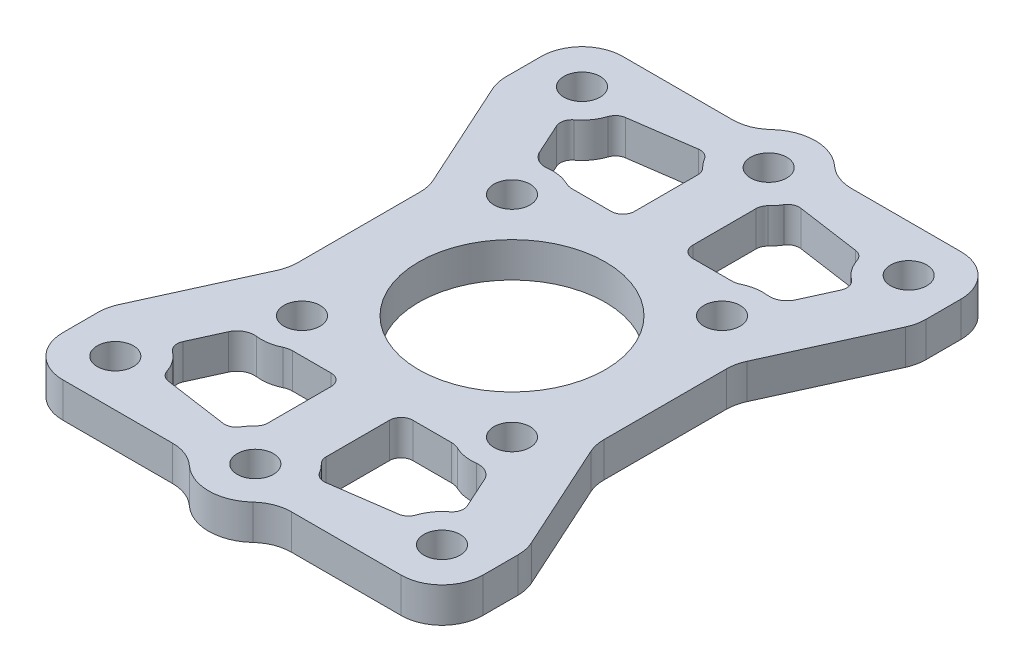
SolidWorks part; units mm, degrees
material "Thornel Mat VMA"
ref_plane "前视基准面" through (0, 0, 0) normal (0, 0, 1) x (1, 0, 0)
ref_plane "上视基准面" through (0, 0, 0) normal (0, 1, 0) x (1, 0, 0)
ref_plane "右视基准面" through (0, 0, 0) normal (1, 0, 0) x (0, 0, -1)
other "Configuration Table"
sketch "草图3" plane through (0, 0, 0) normal (0, 1, 0) x (1, 0, 0)
  line L0 (10, -34.1992) -> (10, 52.6309) construction
  line L1 (0, 0) -> (31.1432, 0) construction
  line L6 (-14, 20) -> (14, 20) construction
  line L7 (-14, 20) -> (-14, -20) construction
  line L8 (-14, -20) -> (14, -20) construction
  line L9 (14, 20) -> (14, -20) construction
  line L10 (-14, 20) -> (14, -20) construction
  line L11 (-14, -20) -> (14, 20) construction
  line L12 (-18, -24) -> (18, -24)
  line L13 (-18, -24) -> (-18, 24)
  line L14 (-18, 24) -> (18, 24)
  line L15 (18, -24) -> (18, 24)
  line L16 (-18, -24) -> (18, 24) construction
  line L17 (-18, 24) -> (18, -24) construction
  line L18 (6, 62.0596) -> (6, -48.8242) construction
  line L19 (0, 0) -> (0, -41.7674) construction
  line L21 (-9, 9) -> (9, 9) construction
  line L22 (-9, 9) -> (-9, -9) construction
  line L23 (-9, -9) -> (9, -9) construction
  line L24 (9, 9) -> (9, -9) construction
  line L25 (-9, 9) -> (9, -9) construction
  line L26 (-9, -9) -> (9, 9) construction
  circle A7 centre (14, 20) radius 1.55
  circle A8 centre (-14, 20) radius 1.55
  circle A9 centre (-14, -20) radius 1.55
  circle A10 centre (14, -20) radius 1.55
  circle A15 centre (0, 22) radius 1.55
  circle A17 centre (0, 22) radius 4
  circle A19 centre (0, -22) radius 1.55
  circle A20 centre (0, -22) radius 4
  circle A30 centre (9, 9) radius 1.55
  circle A31 centre (-9, 9) radius 1.55
  circle A32 centre (-9, -9) radius 1.55
  circle A33 centre (9, -9) radius 1.55
  circle A34 centre (0, 0) radius 8
  point P14 (0, 0)
  point P42 (0, 0)
  dimension "D2" = 6
  dimension "D4" = 16
  dimension "D9" = 3.1
  dimension "D12" = 4
  dimension "D13" = 8
  dimension "D14" = 2
  dimension "D3" = 18
  dimension "D6" = 10
  dimension "D7" = 4
  dimension "D8" = 40
  dimension "D10" = 28
  dimension "D11" = 4
extrude "凸台-拉伸1" add sketch "草图3" along normal blind 3
sketch "草图4" plane through (0, 3, 0) normal (0, 1, 0) x (1, 0, 0)
  line L17 (-14, 20) -> (0, 22) construction
  line L32 (0, 22) -> (14, 20) construction
  line L33 (14, 20) -> (9, 9) construction
  line L34 (9, 9) -> (-9, 9) construction
  line L35 (-9, 9) -> (-14, 20) construction
  line L36 (0, 0) -> (25.4946, 0) construction
  line L37 (0, 0) -> (0, 27.7069) construction
  line L38 (-10.4483, 12.1863) -> (-12.5517, 16.8137)
  line L39 (-10.5382, 19.4844) -> (-3.6926, 20.4623)
  line L40 (10.5382, 19.4844) -> (3.6926, 20.4623)
  line L41 (10.4483, 12.1863) -> (12.5517, 16.8137)
  line L42 (-7.1972, 12) -> (7.1972, 12)
  line L43 (-2.5, 18.8775) -> (-2.5, 12)
  line L44 (2.5, 18.8775) -> (2.5, 12)
  line L45 (-9, -9) -> (-14, -20) construction
  line L46 (9, -9) -> (-9, -9) construction
  line L47 (14, -20) -> (9, -9) construction
  line L48 (0, -22) -> (14, -20) construction
  line L49 (-14, -20) -> (0, -22) construction
  line L50 (2.5, -18.8775) -> (2.5, -12)
  line L51 (-2.5, -18.8775) -> (-2.5, -12)
  line L52 (-7.1972, -12) -> (7.1972, -12)
  line L53 (10.4483, -12.1863) -> (12.5517, -16.8137)
  line L54 (10.5382, -19.4844) -> (3.6926, -20.4623)
  line L55 (-10.5382, -19.4844) -> (-3.6926, -20.4623)
  line L56 (-10.4483, -12.1863) -> (-12.5517, -16.8137)
  line L57 (18, 16.717) -> (13.1287, 6)
  line L58 (18, -24) -> (18, 24) construction
  line L59 (13.1287, 6) -> (13.1287, -6)
  line L60 (13.1287, -6) -> (18, -16.717)
  line L61 (-13.1287, -6) -> (-18, -16.717)
  line L62 (-13.1287, 6) -> (-13.1287, -6)
  line L63 (-18, 16.717) -> (-13.1287, 6)
  line L64 (9, 9) -> (9, -9) construction
  circle A2 centre (-14, 20) radius 3.5
  circle A3 centre (-14, 20) radius 1.55 construction
  circle A4 centre (-9, 9) radius 3.5
  circle A5 centre (0, 22) radius 4
  arc A6 (3.4641, 24) -> (-3.4641, 24) centre (0, 22) ccw construction
  circle A7 centre (9, 9) radius 3.5
  circle A8 centre (14, 20) radius 3.5
  circle A9 centre (14, -20) radius 3.5
  circle A10 centre (9, -9) radius 3.5
  circle A11 centre (0, -22) radius 4
  circle A12 centre (-9, -9) radius 3.5
  circle A13 centre (-14, -20) radius 3.5
  dimension "D1" = 1.95
  dimension "D6" = 1
  dimension "D2" = 3
  dimension "D3" = 5
  dimension "D4" = 5
  dimension "D5" = 12
extrude "切除-拉伸1" cut sketch "草图4" against normal through all and the other way through all
fillet "圆角1" radius 3.5 16 edges at (-18, 1.5, 24) (3.4641, 1.5, 24) (-3.4641, 1.5, 24) (18, 1.5, 24) (18, 1.5, -24) (-3.4641, 1.5, -24) (3.4641, 1.5, -24) (-18, 1.5, -24) (13.1287, 1.5, -6) (13.1287, 1.5, 6) (18, 1.5, 16.717) (-18, 1.5, 16.717) (-13.1287, 1.5, 6) (-13.1287, 1.5, -6) (-18, 1.5, -16.717) (18, 1.5, -16.717)
fillet "圆角6" radius 1 20 edges at (-12.5517, 1.5, -16.8137) (-2.5, 1.5, -12) (-2.5, 1.5, -18.8775) (2.5, 1.5, -18.8775) (12.5517, 1.5, -16.8137) (2.5, 1.5, -12) (-12.5517, 1.5, 16.8137) (-2.5, 1.5, 12) (-2.5, 1.5, 18.8775) (2.5, 1.5, 12) (2.5, 1.5, 18.8775) (3.6926, 1.5, 20.4623) (-3.6926, 1.5, 20.4623) (-10.5382, 1.5, 19.4844) (12.5517, 1.5, 16.8137) (10.5382, 1.5, 19.4844) (10.5382, 1.5, -19.4844) (3.6926, 1.5, -20.4623) (-3.6926, 1.5, -20.4623) (-10.5382, 1.5, -19.4844)
fillet "圆角7" radius 1.5 8 edges at (7.1972, 1.5, 12) (10.4483, 1.5, 12.1863) (10.4483, 1.5, -12.1863) (7.1972, 1.5, -12) (-10.4483, 1.5, -12.1863) (-7.1972, 1.5, -12) (-10.4483, 1.5, 12.1863) (-7.1972, 1.5, 12)
